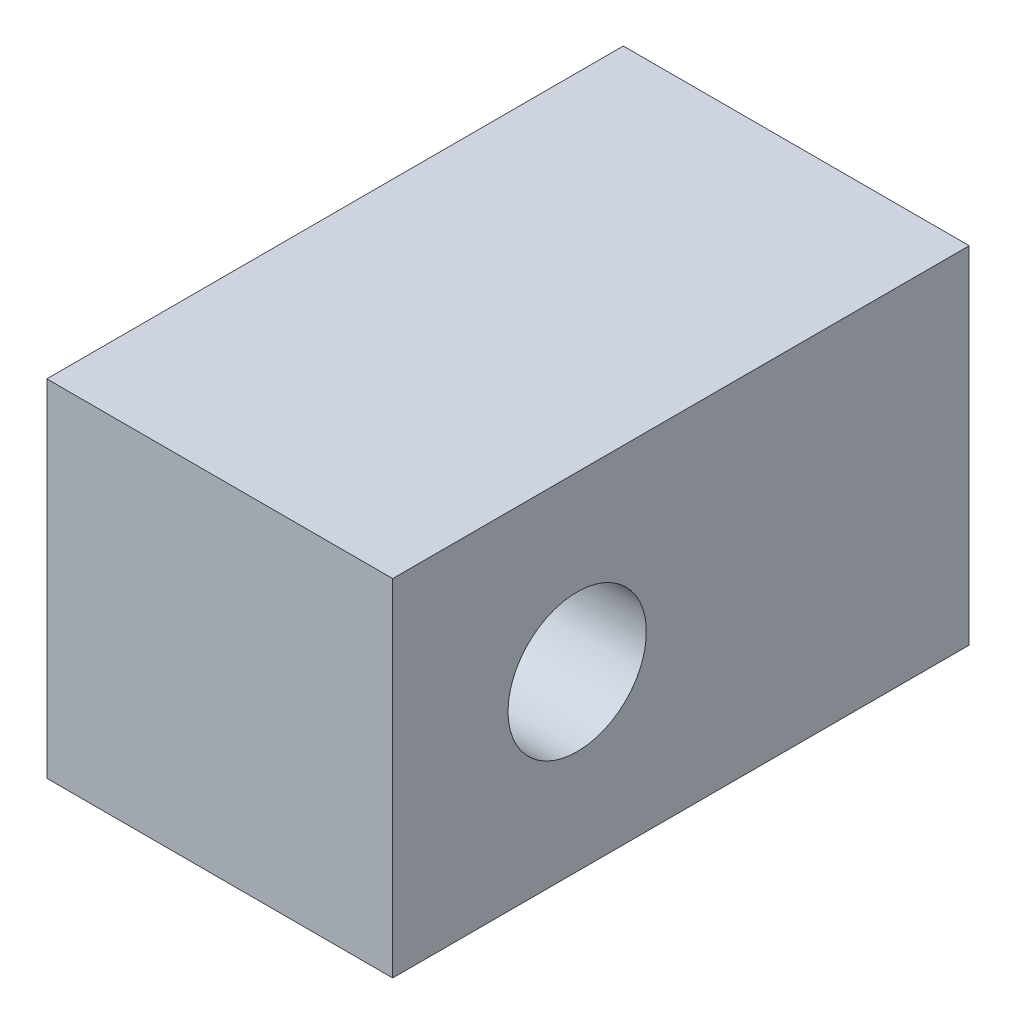
SolidWorks part; units mm, degrees
ref_plane "Front Plane" through (0, 0, 0) normal (0, 0, 1) x (1, 0, 0)
ref_plane "Top Plane" through (0, 0, 0) normal (0, 1, 0) x (1, 0, 0)
ref_plane "Right Plane" through (0, 0, 0) normal (1, 0, 0) x (0, 0, -1)
sketch "Sketch1" plane through (0, 0, 0) normal (0, 0, 1) x (1, 0, 0)
  line L1 (-7.5, 7.5) -> (7.5, 7.5)
  line L2 (-7.5, 7.5) -> (-7.5, -7.5)
  line L3 (-7.5, -7.5) -> (7.5, -7.5)
  line L4 (7.5, 7.5) -> (7.5, -7.5)
  line L5 (-7.5, 7.5) -> (7.5, -7.5) construction
  line L6 (-7.5, -7.5) -> (7.5, 7.5) construction
  point P0 (0, 0)
  dimension "D1" = 15
  dimension "D2" = 15
extrude "Boss-Extrude1" add sketch "Sketch1" along normal blind 25
sketch "Sketch2" plane through (-7.5, 0, 0) normal (-1, 0, 0) x (0, 0, 1)
  line L0 (0, 0) -> (28.5329, 0) construction
  line L1 (25, 7.5) -> (25, -7.5) construction
  circle A0 centre (17, 0) radius 3
  dimension "D1" = 6
  dimension "D2" = 8
extrude "Cut-Extrude1" cut sketch "Sketch2" against normal through all both and the other way through all
